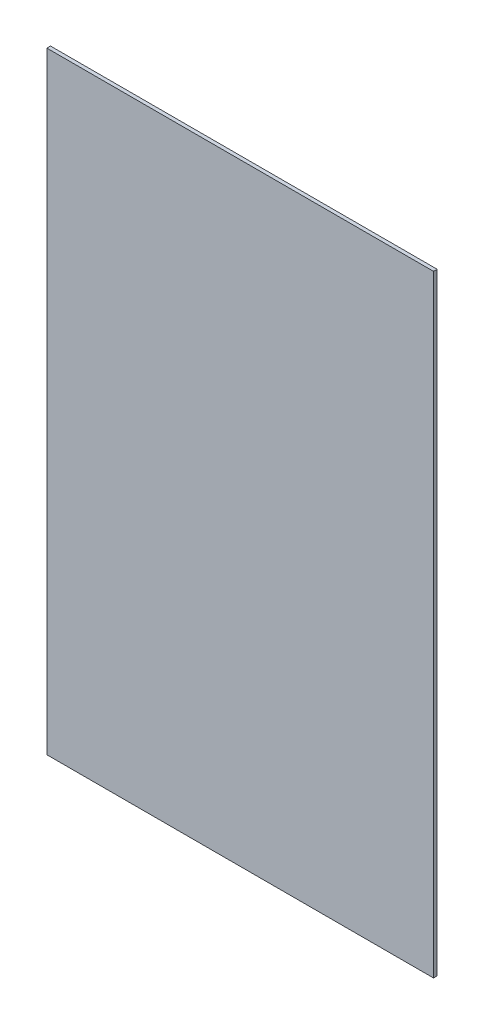
from build123d import *

# Parameters (mm, degrees)
SKETCH_1_W      = 532
SKETCH_1_H      = 842
EXTRUDE_1_DEPTH = 5


with BuildPart() as part:
    # 草图1 → 凸台-拉伸1 (new body)
    with BuildSketch(Plane.XY):
        Rectangle(SKETCH_1_W, SKETCH_1_H)
    extrude(amount=EXTRUDE_1_DEPTH)


solid = part.part
